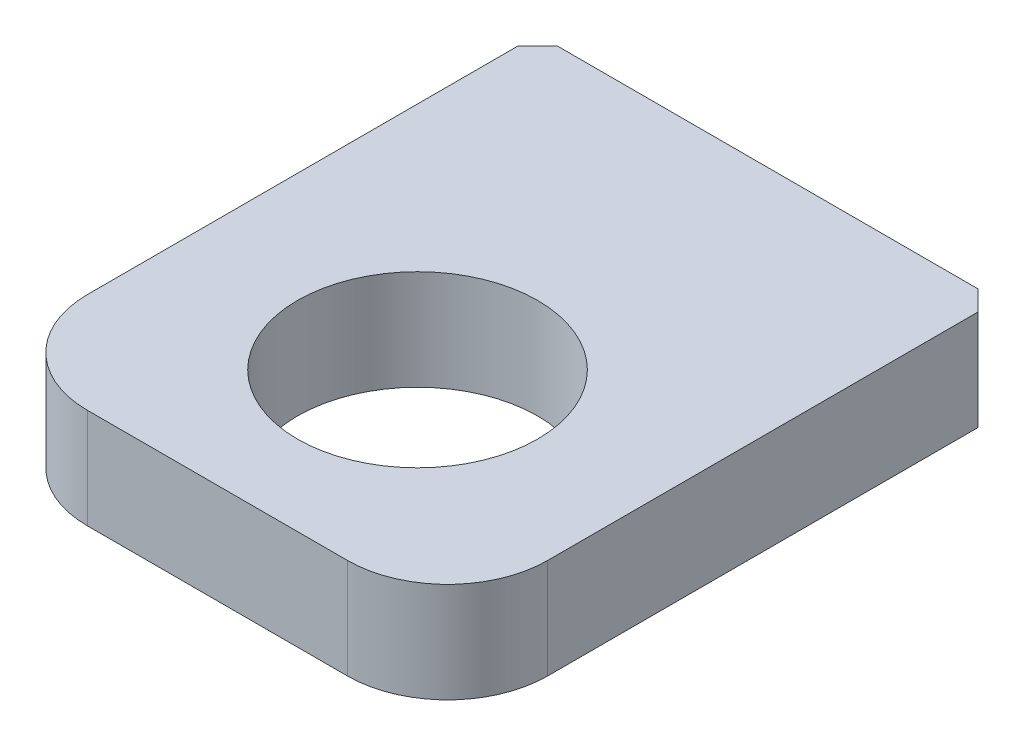
from build123d import *

# Parameters (mm, degrees)
SKETCH_1_W             = 46
SKETCH_1_H             = 55
EXTRUDE_1_DEPTH        = 5
HOLE_WIZARD_M27_1_0_D  = 24
FILLET_1_R             = 10
HOLE_WIZARD_M4_1_D     = 3.3
HOLE_WIZARD_M4_1_DEPTH = 11.5
HOLE_WIZARD_M4_1_TIP   = 0.991420021
CHAMFER_1_SIZE         = 2


with BuildPart() as part:
    # 草图1 → 凸台-拉伸1 (new, symmetric)
    with BuildSketch(Plane(origin=(0, 0, 0), x_dir=(1, 0, 0), z_dir=(0, 1, 0))):
        Rectangle(SKETCH_1_W, SKETCH_1_H)
    extrude(amount=EXTRUDE_1_DEPTH, both=True)

    # M27*1.0反牙 (through all)
    with Locations(Plane(origin=(0, 5, 0), x_dir=(1, 0, 0), z_dir=(0, 1, 0))):
        with Locations((0, -7.5)):
            Hole(HOLE_WIZARD_M27_1_0_D / 2)

    # 圆角1
    fillet_1_edges = [part.edges().sort_by_distance(p)[0] for p in [
        (23, 0, 27.5),
        (-23, 0, 27.5),
    ]]
    fillet(fillet_1_edges, radius=FILLET_1_R)

    # M4 螺纹孔1
    with Locations(Plane(origin=(0, 0, -27.5), x_dir=(-1, 0, 0), z_dir=(0, 0, -1))):
        with Locations((-15, 0), (15, 0)):
            Hole(HOLE_WIZARD_M4_1_D / 2, depth=HOLE_WIZARD_M4_1_DEPTH)
            with Locations((0, 0, -(HOLE_WIZARD_M4_1_DEPTH + HOLE_WIZARD_M4_1_TIP / 2))):  # 118° drill point
                Cone(0, HOLE_WIZARD_M4_1_D / 2, HOLE_WIZARD_M4_1_TIP, mode=Mode.SUBTRACT)

    # 倒角1
    chamfer_1_edges = [part.edges().sort_by_distance(p)[0] for p in [
        (-23, 0, -27.5),
        (23, 0, -27.5),
    ]]
    chamfer(chamfer_1_edges, length=CHAMFER_1_SIZE)


solid = part.part
